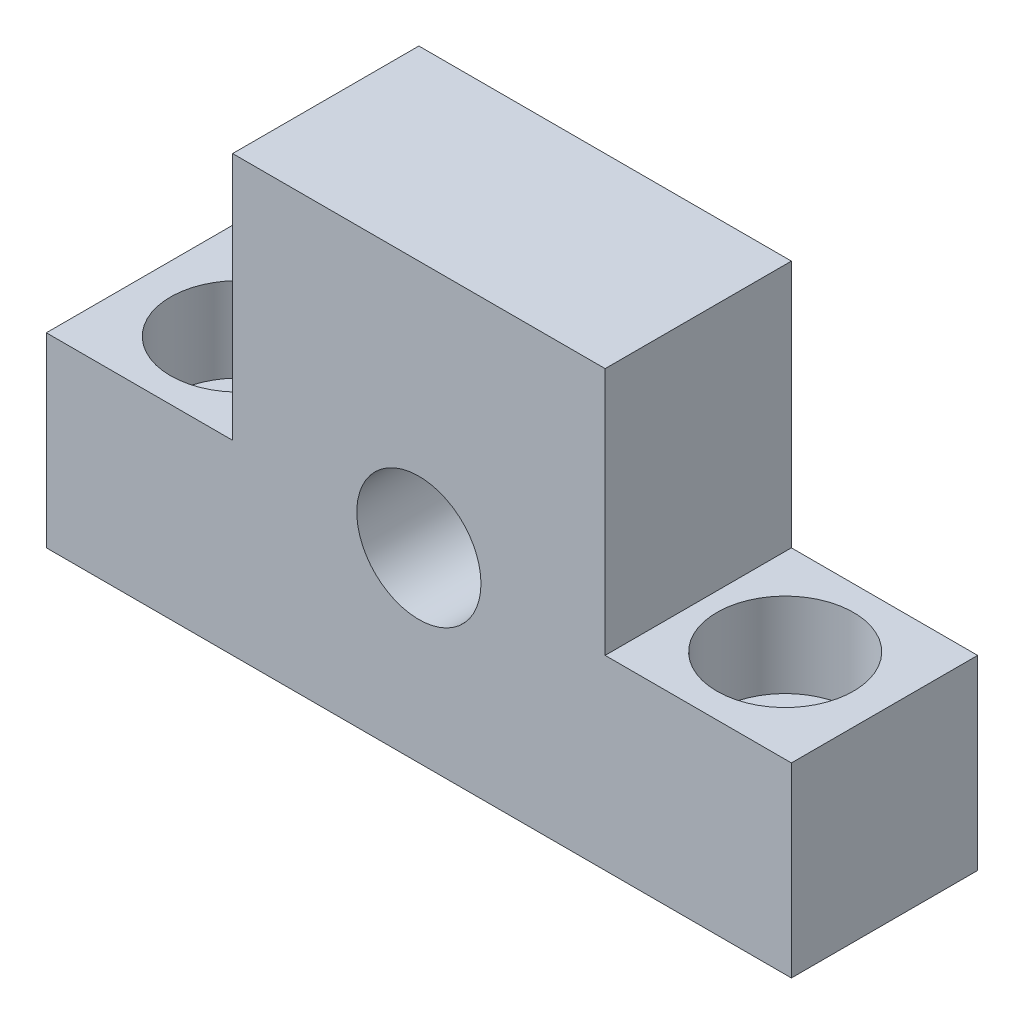
from build123d import *

# Parameters (mm, degrees)
BOSS_EXTRUDE1_DEPTH                                  = 15
SKETCH2_R                                            = 5
CUT_EXTRUDE1_DEPTH                                   = 72.063352018
CBORE_FOR_M6_HEXAGON_SOCKET_HEAD_CAP_SCR_D           = 6.6
CBORE_FOR_M6_HEXAGON_SOCKET_HEAD_CAP_SCR_CBORE_D     = 11
CBORE_FOR_M6_HEXAGON_SOCKET_HEAD_CAP_SCR_CBORE_DEPTH = 6.8


with BuildPart() as part:
    # Sketch1 → Boss-Extrude1 (new body)
    with BuildSketch(Plane.XY):
        Polygon((0, 0), (0, 15), (15, 15), (15, 35), (45, 35), (45, 15), (60, 15), (60, 0), align=None)
    extrude(amount=BOSS_EXTRUDE1_DEPTH)

    # Sketch2 → Cut-Extrude1 (cut, through all)
    with BuildSketch(Plane.XY.offset(15)):
        with Locations((30, 15)):
            Circle(SKETCH2_R)
    extrude(amount=-CUT_EXTRUDE1_DEPTH, mode=Mode.SUBTRACT)

    # CBORE for M6 Hexagon socket head cap screws1 (through all)
    with Locations(Plane(origin=(8, 15, 7.5), x_dir=(0, 0, 1), z_dir=(0, 1, 0))):
        with Locations((0, 0), (0, 44)):
            CounterBoreHole(CBORE_FOR_M6_HEXAGON_SOCKET_HEAD_CAP_SCR_D / 2, CBORE_FOR_M6_HEXAGON_SOCKET_HEAD_CAP_SCR_CBORE_D / 2, CBORE_FOR_M6_HEXAGON_SOCKET_HEAD_CAP_SCR_CBORE_DEPTH)


solid = part.part
